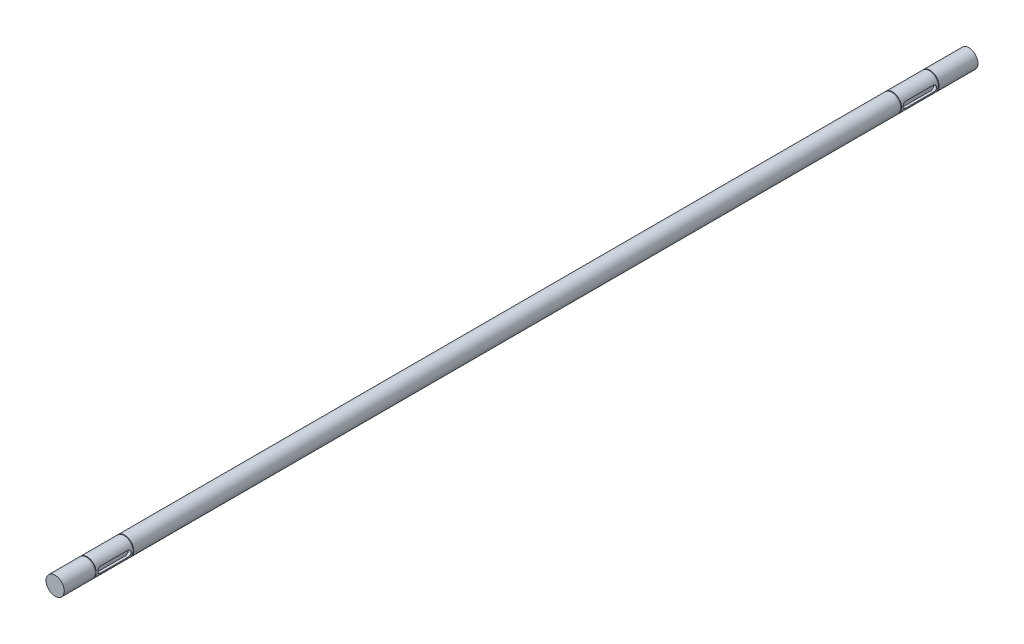
SolidWorks part; units mm, degrees
ref_plane "前视基准面" through (0, 0, 0) normal (0, 0, 1) x (1, 0, 0)
ref_plane "上视基准面" through (0, 0, 0) normal (0, 1, 0) x (1, 0, 0)
ref_plane "右视基准面" through (0, 0, 0) normal (1, 0, 0) x (0, 0, -1)
sketch "草图2" plane through (0, 0, 0) normal (0, 0, 1) x (1, 0, 0)
  circle A0 centre (0, 0) radius 15
  dimension "D1" = 30
extrude "凸台-拉伸1" add sketch "草图2" along normal blind 1500
ref_plane "基准面1" through (10, 0, 0) normal (1, 0, 0) x (0, 0, -1)
sketch "草图3" plane through (10, 0, 0) normal (1, 0, 0) x (0, 0, -1)
  line L0 (-1440, 0) -> (-1395, 0) construction
  line L1 (-1440, 5) -> (-1395, 5)
  line L2 (-1440, -5) -> (-1395, -5)
  line L3 (-73, 0) -> (-118, 0) construction
  line L4 (-73, -5) -> (-118, -5)
  line L5 (-73, 5) -> (-118, 5)
  line L6 (-1500, 0) -> (-1298.0298, 0) construction
  line L7 (-1500, 15) -> (-1500, -15) construction
  line L8 (-756.5, -15) -> (-756.5, 82.1369) construction
  arc A0 (-1440, 5) -> (-1440, -5) centre (-1440, 0) ccw
  arc A1 (-1395, -5) -> (-1395, 5) centre (-1395, 0) ccw
  arc A2 (-73, -5) -> (-73, 5) centre (-73, 0) ccw
  arc A3 (-118, 5) -> (-118, -5) centre (-118, 0) ccw
  point P2 (-1417.5, 0)
  point P8 (-95.5, 0)
  dimension "D1" = 45
  dimension "D2" = 10
  dimension "D3" = 1322
  dimension "D4" = 743.5
extrude "切除-拉伸1" cut sketch "草图3" along normal through all
sketch "草图4" plane through (0, 0, 0) normal (1, 0, 0) x (0, 0, -1)
  line L0 (0, 15) -> (-1500, 15) construction
  line L1 (-1449.1, 15) -> (-1447.5, 15)
  line L2 (-1449.1, 15) -> (-1449.1, 14.3)
  line L3 (-1449.1, 14.3) -> (-1447.5, 14.3)
  line L4 (-1447.5, 15) -> (-1447.5, 14.3)
  line L5 (-1417.5, -5) -> (-1417.5, 24.0229) construction
  line L6 (-1387.5, 15) -> (-1385.9, 15)
  line L7 (-1387.5, 15) -> (-1387.5, 14.3)
  line L8 (-1387.5, 14.3) -> (-1385.9, 14.3)
  line L9 (-1385.9, 15) -> (-1385.9, 14.3)
  line L10 (-1440, -5) -> (-1395, -5) construction
  line L11 (-1445, 0) -> (-1566.2273, 0) construction
  arc A0 (-1440, 5) -> (-1440, -5) centre (-1440, 0) ccw construction
  arc A1 (-1440, 5) -> (-1440, -5) centre (-1440, 0) ccw construction
  dimension "D1" = 1.6
  dimension "D2" = 14.3
  dimension "D3" = 60
revolve "切除-旋转5" cut sketch "草图4" angle 360 about L11
pattern_linear "阵列(线性)1" count 2 spacing 1322 along (0, 0, -1) of "切除-旋转5"
hole_wizard "M8 螺纹孔1" positions "草图5" profile "草图6" tap size "M8" standard "GB"
sketch "草图5" plane through (0, 0, 0) normal (0, 0, -1) x (-1, 0, 0)
  point P0 (0, 0)
sketch "草图6" plane through (0, 0, 0) normal (1, 0, 0) x (0, 1, 0)
  line L0 (0, 0) -> (0, 21.7929)
  line L1 (0, 21.7929) -> (3.4, 19.75)
  line L2 (3.4, 19.75) -> (3.4, 0)
  line L5 (3.4, 0) -> (0, 0)
  line L10 (0, 21.7929) -> (-3.4, 19.75) construction
  line L11 (0, -6.35) -> (0, 107.95) construction
  dimension "螺纹孔钻头直径" = 6.8
  dimension "螺纹孔钻头深度" = 19.75
  dimension "导头角度" = 118
cosmetic thread "孔螺蚊线1" parameters "D1"=16, "D2"=8
